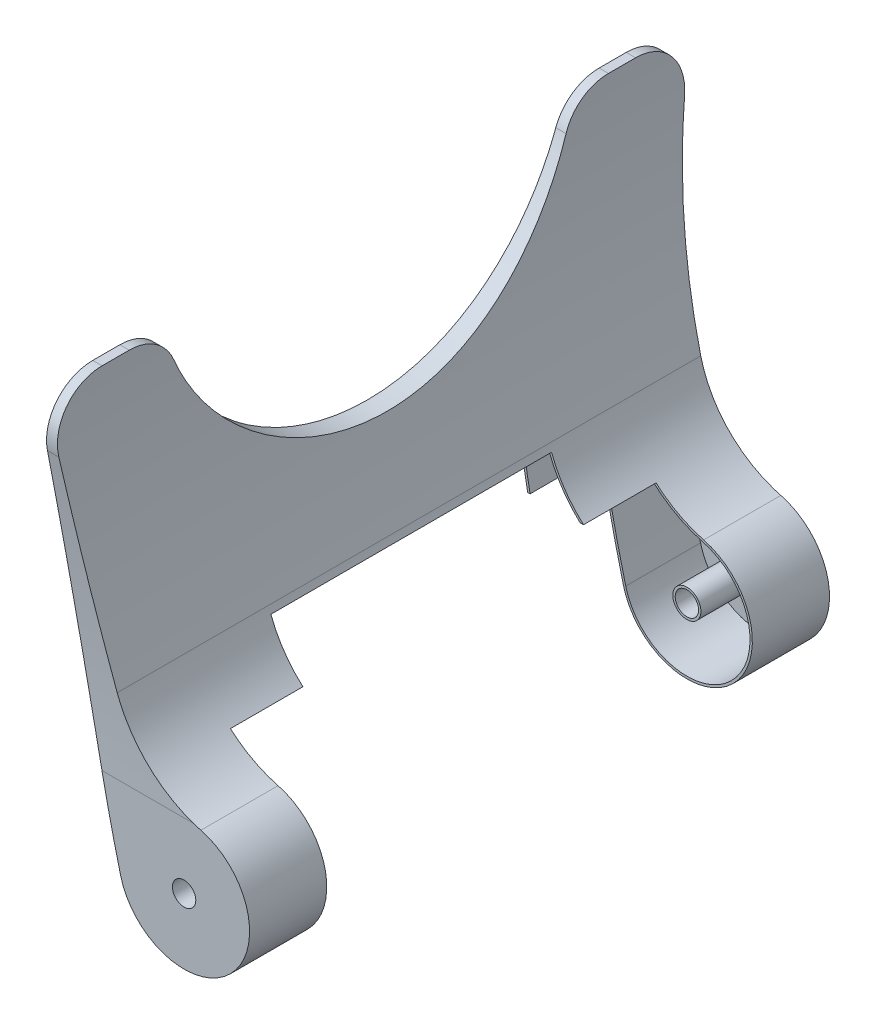
SolidWorks part; units mm, degrees
ref_plane "Front Plane" through (0, 0, 0) normal (0, 0, 1) x (1, 0, 0)
ref_plane "Top Plane" through (0, 0, 0) normal (0, 1, 0) x (1, 0, 0)
ref_plane "Right Plane" through (0, 0, 0) normal (1, 0, 0) x (0, 0, -1)
sketch "Sketch1" plane through (0, 0, 0) normal (0, 0, 1) x (1, 0, 0)
  line L0 (-49, 168) -> (-45, 168)
  arc A1 (-27.1249, -6.9453) -> (-49, 168) centre (650.9988, 166.6871) cw
  arc A3 (-45, 168) -> (-27.8424, 60.8627) centre (354.8965, 177.0995) ccw
  arc A4 (-27.8424, 60.8627) -> (7.1795, 27.0639) centre (20, 75.3923) ccw
  arc A5 (-27.1249, -6.9453) -> (7.1795, 27.0639) centre (0, 0) ccw
  dimension "D1" = 56
  dimension "D2" = 700
  dimension "D3" = 45
  dimension "D5" = 400
  dimension "D7" = 50
  dimension "D4" = 168
  dimension "D6" = 4
  dimension "D8" = 20
extrude "Boss-Extrude1" add sketch "Sketch1" along normal mid plane 300
sketch "Sketch2" plane through (0, 0, 0) normal (1, 0, 0) x (0, 0, -1)
  line L0 (-150, 168) -> (150, 168) construction
  line L2 (-114.0704, 168) -> (-102.4695, 168)
  line L3 (-121, -8) -> (121, -8) construction
  line L4 (102.4695, 168) -> (114.0704, 168)
  line L5 (-150, -28) -> (150, -28) construction
  line L6 (124, -8) -> (124, -28)
  line L7 (0, 42.3507) -> (0, -42.3507) construction
  line L8 (-150, -28) -> (150, -28) construction
  line L9 (-124, 28) -> (-124, -8)
  line L12 (-150, 168) -> (150, 168)
  line L13 (124, 28) -> (124, -8)
  line L15 (-124, -8) -> (-121, -8)
  line L16 (-121, -8) -> (-121, 12)
  line L17 (-121, 12) -> (-91, 12)
  line L18 (-91, 12) -> (-91, 32)
  line L19 (-91, 32) -> (91, 32)
  line L20 (124, -8) -> (121, -8)
  line L21 (121, -8) -> (121, 12)
  line L22 (121, 12) -> (91, 12)
  line L23 (91, 12) -> (91, 32)
  line L24 (-150, 168) -> (-150, -28)
  line L25 (-150, -28) -> (150, -28)
  line L26 (150, 168) -> (150, -28)
  line L27 (-124, -8) -> (-124, -28)
  arc A0 (-114.0704, 168) -> (-133.7907, 144.6667) centre (-114.0704, 148) ccw
  arc A1 (-102.4695, 168) -> (-83.8387, 155.2727) centre (-102.4695, 148) cw
  arc A2 (-83.8387, 155.2727) -> (83.8387, 155.2727) centre (0, 188) ccw
  arc A3 (-133.7907, 144.6667) -> (-124, 28) centre (-824, 28) cw
  arc A4 (133.7907, 144.6667) -> (124, 28) centre (824, 28) ccw
  arc A5 (114.0704, 168) -> (133.7907, 144.6667) centre (114.0704, 148) cw
  arc A6 (102.4695, 168) -> (83.8387, 155.2727) centre (102.4695, 148) ccw
  point P45 (0, 32)
  dimension "D1" = 20
  dimension "D2" = 90
  dimension "D5" = 124
  dimension "D7" = 20
  dimension "D3" = 700
  dimension "D8" = 20
  dimension "D4" = 56
  dimension "D6" = 216
  dimension "D9" = 56
  dimension "D10" = 3
  dimension "D11" = 91
  dimension "D12" = 20
  dimension "D13" = 20
extrude "Cut-Extrude5" cut sketch "Sketch2" against normal mid plane 203 contours A3 A0 L12 L24 L25 L27 L9 | A6 L12 A1 A2 | L12 A5 A4 L13 L6 L25 L26
sketch "Sketch3" plane through (0, 0, 124) normal (0, 0, 1) x (1, 0, 0)
  circle A0 centre (0, 0) radius 5
  dimension "D1" = 10
extrude "Cut-Extrude6" cut sketch "Sketch3" against normal blind 277
sketch "Sketch4" plane through (0, 0, 0) normal (1, 0, 0) x (0, 0, -1)
  line L0 (-124, -28) -> (-91, -28)
  line L2 (-124, -28) -> (124, -28) construction
  line L3 (-91, -28) -> (-91, 38)
  line L4 (-91, 38) -> (-60, 38)
  line L5 (-60, 38) -> (-60, 58)
  line L6 (-60, 58) -> (60, 58)
  line L7 (0, 42.3507) -> (0, -42.3507) construction
  line L10 (91, -28) -> (91, 38)
  line L11 (91, 38) -> (60, 38)
  line L12 (60, 38) -> (60, 58)
  line L13 (-91, -28) -> (91, -28)
  point P15 (0, 58)
  dimension "D1" = 91
  dimension "D2" = 60
  dimension "D3" = 66
  dimension "D4" = 20
extrude "Cut-Extrude8" cut sketch "Sketch4" against normal mid plane 277 contours L3 L13 L10 L11 L12 L6 L5 L4
shell "Shell1" thickness 1
